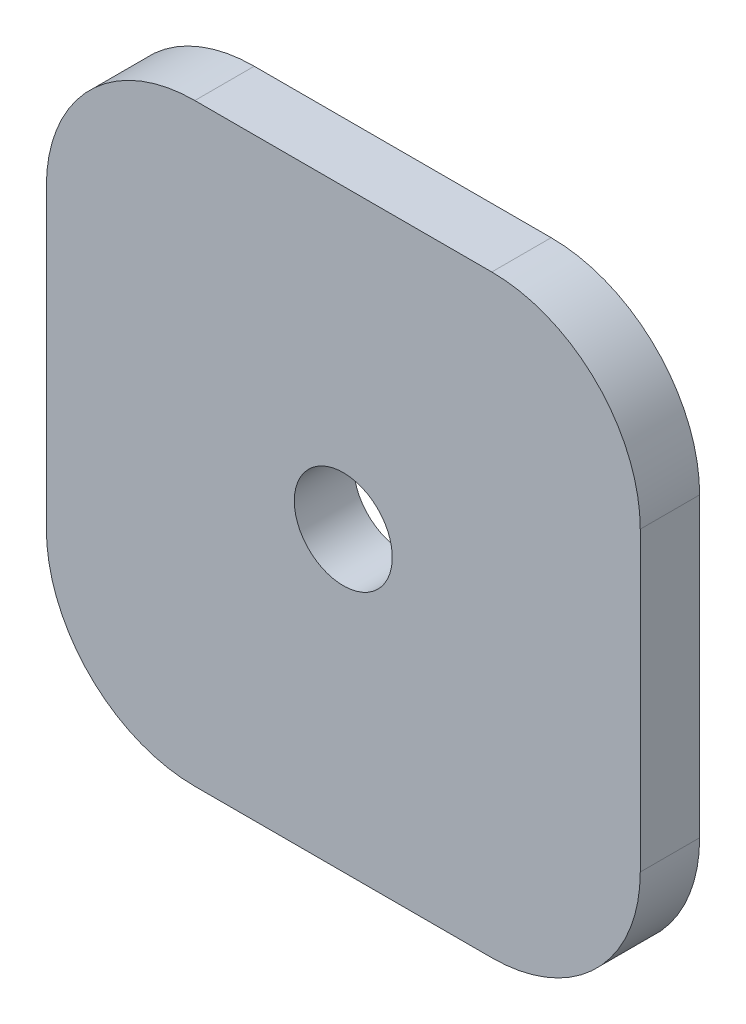
from build123d import *

# Parameters (mm, degrees)
SKETCH_1_W         = 40
SKETCH_1_H         = 40
EXTRUDE_1_DEPTH    = 4
FILLET_1_R         = 10
HOLE_WIZARD_M6_1_D = 6.6


with BuildPart() as part:
    # 草图1 → 凸台-拉伸1 (new body)
    with BuildSketch(Plane.XY):
        Rectangle(SKETCH_1_W, SKETCH_1_H)
    extrude(amount=EXTRUDE_1_DEPTH)

    # 圆角1
    fillet_1_edges = [part.edges().sort_by_distance(p)[0] for p in [
        (20, -20, 2),
        (-20, -20, 2),
        (-20, 20, 2),
        (20, 20, 2),
    ]]
    fillet(fillet_1_edges, radius=FILLET_1_R)

    # Hole Wizard M6 _1 (through all)
    with Locations(Plane(origin=(0, 0, 0), x_dir=(-1, 0, 0), z_dir=(0, 0, -1))):
        with Locations((0, 0)):
            Hole(HOLE_WIZARD_M6_1_D / 2)


solid = part.part
